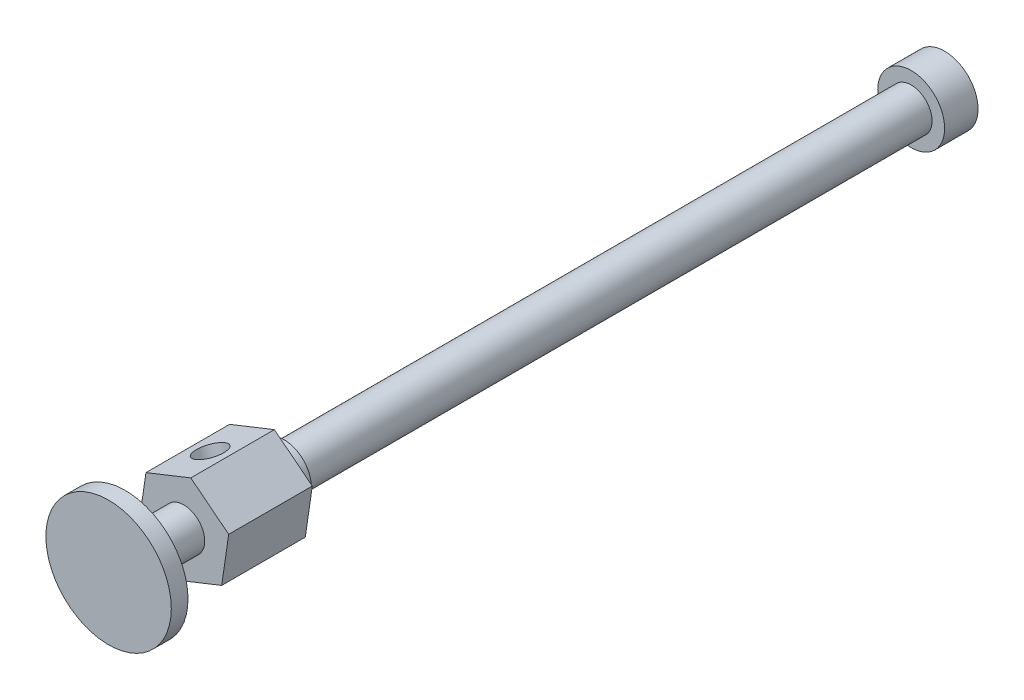
SolidWorks part; units mm, degrees
ref_plane "Front Plane" through (0, 0, 0) normal (0, 0, 1) x (1, 0, 0)
ref_plane "Top Plane" through (0, 0, 0) normal (0, 1, 0) x (1, 0, 0)
ref_plane "Right Plane" through (0, 0, 0) normal (1, 0, 0) x (0, 0, -1)
other "Configuration Table"
sketch "Sketch1" plane through (0, 0, 0) normal (0, 0, 1) x (1, 0, 0)
  line L0 (0, 3.2171) -> (0, -3.2171) construction
  point P4 (0, 0)
sketch "Sketch2" plane through (0, 0, 0) normal (0, 0, 1) x (1, 0, 0)
  circle A0 centre (20.6091, -9.3107) radius 2.5
  dimension "D1" = 5
extrude "Boss-Extrude1" add sketch "Sketch2" along normal blind 100
sketch "Sketch3" plane through (0, 0, 0) normal (0, 0, -1) x (-1, 0, 0)
  circle A0 centre (-20.6091, -9.3107) radius 4
  dimension "D1" = 8
extrude "Boss-Extrude2" add sketch "Sketch3" against normal blind 4
sketch "Sketch4" plane through (0, 0, 100) normal (0, 0, 1) x (1, 0, 0)
  circle A0 centre (20.6091, -9.3107) radius 7.5
  dimension "D1" = 15
extrude "Boss-Extrude3" add sketch "Sketch4" against normal blind 2
ref_plane "Plane1" through (0, 0, 91) normal (0, 0, -1) x (-1, 0, 0)
sketch "Sketch5" plane through (0, 0, 91) normal (0, 0, -1) x (-1, 0, 0)
  line L1 (-16.0795, -5.7307) -> (-21.4446, -3.598)
  line L2 (-21.4446, -3.598) -> (-25.9742, -7.178)
  line L3 (-25.9742, -7.178) -> (-25.1386, -12.8907)
  line L4 (-25.1386, -12.8907) -> (-19.7735, -15.0234)
  line L5 (-19.7735, -15.0234) -> (-15.2439, -11.4434)
  line L6 (-15.2439, -11.4434) -> (-16.0795, -5.7307)
  circle A0 centre (-20.6091, -9.3107) radius 5 construction
  dimension "D1" = 10
extrude "Boss-Extrude4" add sketch "Sketch5" along normal blind 10
sketch "Sketch6" plane through (0, 0, 81) normal (0, 0, -1) x (-1, 0, 0)
  circle A0 centre (-20.6091, -9.3107) radius 3.25
  dimension "D1" = 6.5
extrude "Boss-Extrude5" add sketch "Sketch6" along normal blind 2
sketch "Sketch7" plane through (4.1614, -10.4684, 0) normal (-0.3694, 0.9293, 0) x (0.9293, 0.3694, 0)
  line L0 (15.712, -81) -> (15.712, -91) construction
  line L1 (12.8252, -81) -> (18.5987, -81) construction
  line L2 (12.8252, -91) -> (18.5987, -91) construction
  circle A0 centre (15.712, -86) radius 1.75
  dimension "D1" = 3.5
extrude "Cut-Extrude1" cut sketch "Sketch7" against normal blind 2
